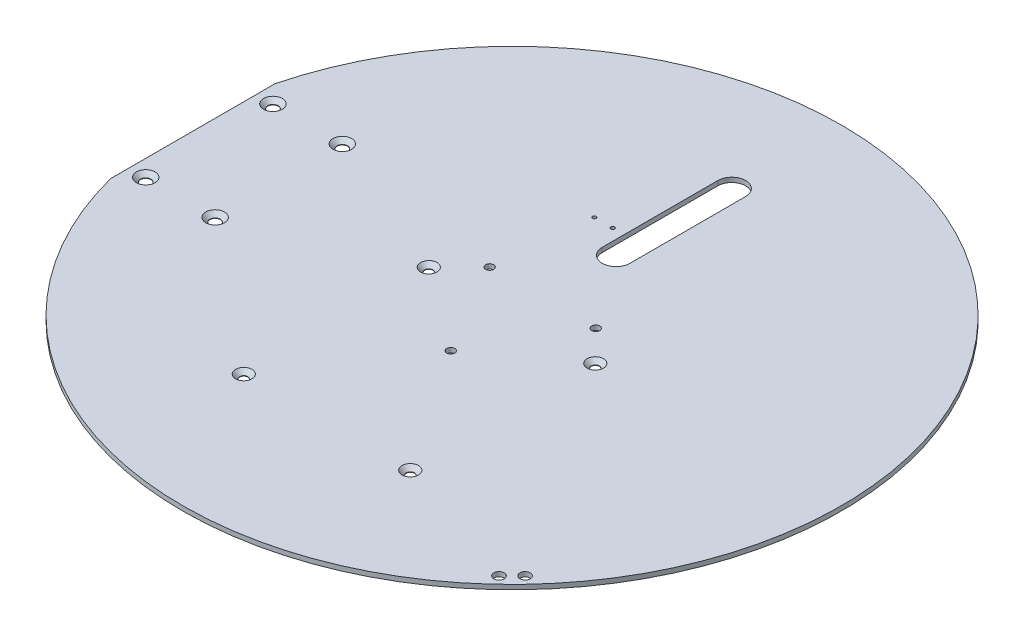
from build123d import *

# Parameters (mm, degrees)
SKETCH1_R             = 142.5
BOSS_EXTRUDE1_DEPTH   = 2
SKETCH3_R             = 1.75
CUT_EXTRUDE1_DEPTH    = 10
CIRPATTERN1_COUNT     = 3
SKETCH5_R             = 2.25
CUT_EXTRUDE2_DEPTH    = 10
CUT_EXTRUDE3_DEPTH    = 202.5353567
SKETCH7_R             = 1.75
CUT_EXTRUDE4_DEPTH    = 10
CHAMFER1_SIZE         = 1.8
CHAMFER2_SIZE         = 1.8
M2_TAPPED_HOLE1_D     = 1.6
M2_TAPPED_HOLE1_DEPTH = 5.2
M2_TAPPED_HOLE1_TIP   = 0.480688495
SKETCH9_W             = 15.607073654
SKETCH9_H             = 79.285494628
CUT_EXTRUDE5_DEPTH    = 10


with BuildPart() as part:
    # Sketch1 → Boss-Extrude1 (new body)
    with BuildSketch(Plane(origin=(0, 0, 0), x_dir=(1, 0, 0), z_dir=(0, 1, 0))):
        with Locations(Location((0, 0, 0), (0, 0, 270))):
            Circle(SKETCH1_R)
    extrude(amount=BOSS_EXTRUDE1_DEPTH)

    # Sketch3 → Cut-Extrude1 (cut)
    with BuildSketch(Plane(origin=(0, 2, 0), x_dir=(1, 0, 0), z_dir=(0, 1, 0))):
        with Locations(Location((0, -26.5, 0), (0, 0, 270))):
            Circle(SKETCH3_R)
    cut_extrude1 = extrude(amount=-CUT_EXTRUDE1_DEPTH, mode=Mode.SUBTRACT)

    # CirPattern1: Cut-Extrude1 ×3 about axis
    cirpattern1_axis = Axis((0, 0, 0), (0, 1, 0))
    for i in range(1, CIRPATTERN1_COUNT):
        add(cut_extrude1.rotate(cirpattern1_axis, i * 360 / CIRPATTERN1_COUNT), mode=Mode.SUBTRACT)

    # Sketch5 → Cut-Extrude2 (cut)
    with BuildSketch(Plane(origin=(0, 2, 0), x_dir=(1, 0, 0), z_dir=(0, 1, 0))):
        with Locations(Location((94.711308368, -100.368162618, 0), (0, 0, 270))):
            Circle(SKETCH5_R)
        with Locations(Location((100.368162618, -94.711308368, 0), (0, 0, 270))):
            Circle(SKETCH5_R)
        with Locations(Location((-130.892369907, 27.5, 0), (0, 0, 270))):
            Circle(SKETCH5_R)
        with Locations(Location((-130.892369907, -27.5, 0), (0, 0, 270))):
            Circle(SKETCH5_R)
        with Locations(Location((-100.892369907, -27.5, 0), (0, 0, 270))):
            Circle(SKETCH5_R)
        with Locations(Location((-100.892369907, 27.5, 0), (0, 0, 270))):
            Circle(SKETCH5_R)
    extrude(amount=-CUT_EXTRUDE2_DEPTH, mode=Mode.SUBTRACT)

    # Sketch6 → Cut-Extrude3 (cut, through all)
    with BuildSketch(Plane(origin=(0, 2, 0), x_dir=(1, 0, 0), z_dir=(0, 1, 0))):
        with BuildLine():
            Line((-6, 45), (-6, 95))
            ThreePointArc((-6, 95), (0, 101), (6, 95))
            Line((6, 95), (6, 45))
            ThreePointArc((6, 45), (0, 39), (-6, 45))
        make_face()
    extrude(amount=-CUT_EXTRUDE3_DEPTH, mode=Mode.SUBTRACT)

    # Sketch7 → Cut-Extrude4 (cut)
    with BuildSketch(Plane.XZ):
        with Locations(Location((36, 0, 0), (0, 0, 270))):
            Circle(SKETCH7_R)
        with Locations(Location((-36, 0, 0), (0, 0, 270))):
            Circle(SKETCH7_R)
        with Locations(Location((-36, 80, 0), (0, 0, 270))):
            Circle(SKETCH7_R)
        with Locations(Location((36, 80, 0), (0, 0, 270))):
            Circle(SKETCH7_R)
    extrude(amount=-CUT_EXTRUDE4_DEPTH, mode=Mode.SUBTRACT)

    # Chamfer1
    chamfer1_edges = [part.edges().sort_by_distance(p)[0] for p in [
        (36, 2, 1.75),
        (-36, 2, 1.75),
        (-36, 2, 81.75),
        (36, 2, 81.75),
    ]]
    chamfer(chamfer1_edges, length=CHAMFER1_SIZE)

    # Chamfer2
    chamfer2_edges = [part.edges().sort_by_distance(p)[0] for p in [
        (-130.892369907, 2, -29.75),
        (-130.892369907, 2, 25.25),
        (-100.892369907, 2, 25.25),
        (-100.892369907, 2, -29.75),
    ]]
    chamfer(chamfer2_edges, length=CHAMFER2_SIZE)

    # M2 Tapped Hole1
    with Locations(Plane(origin=(-10.95, 0, -54.5), x_dir=(0, 0, -1), z_dir=(0, -1, 0))):
        with Locations((0, 0), (0, -8)):
            Hole(M2_TAPPED_HOLE1_D / 2, depth=M2_TAPPED_HOLE1_DEPTH)
            with Locations((0, 0, -(M2_TAPPED_HOLE1_DEPTH + M2_TAPPED_HOLE1_TIP / 2))):  # 118° drill point
                Cone(0, M2_TAPPED_HOLE1_D / 2, M2_TAPPED_HOLE1_TIP, mode=Mode.SUBTRACT)

    # Sketch9 → Cut-Extrude5 (cut)
    with BuildSketch(Plane(origin=(0, 2, 0), x_dir=(1, 0, 0), z_dir=(0, 1, 0))):
        with Locations((-145.803536827, 0)):
            Rectangle(SKETCH9_W, SKETCH9_H)
    extrude(amount=-CUT_EXTRUDE5_DEPTH, mode=Mode.SUBTRACT)


solid = part.part
